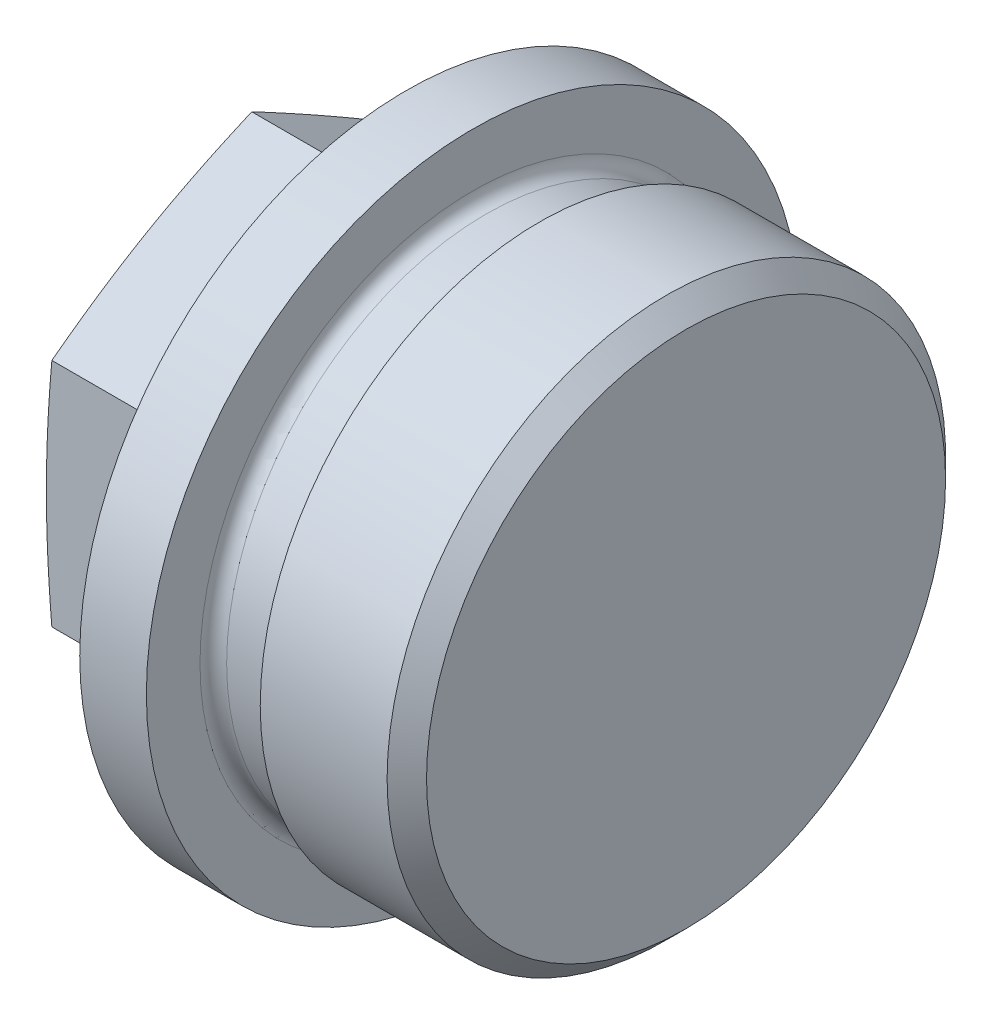
from build123d import *

# Parameters (mm, degrees)
EXTRUDE1_DEPTH     = 12
SKETCH3_OUTSIDE_W  = 179.776
SKETCH3_OUTSIDE_H  = 179.776
SKETCH3_OUTSIDE_R  = 15
CUT_EXTRUDE1_DEPTH = 10
CUT_EXTRUDE1_DRAFT = -80
FILLET1_R          = 1


with BuildPart() as part:
    # Sketch1 → Revolve1 (revolve)
    with BuildSketch(Plane.XY, mode=Mode.PRIVATE) as revolve1_sk:
        Polygon((22, 20.955), (22, 19.476), (17, 19.476), (17, 24.5), (12, 24.5), (12, 1.5), (0, 1.5), (0, 0), (33, 0), (33, 19.476), (31.521, 20.955), align=None)
    revolve(revolve1_sk.sketch.rotate(Axis((0, 0, 0), (1, 0, 0)), 90), axis=Axis((0, 0, 0), (1, 0, 0)))

    # Sketch2 → Extrude1 (add)
    with BuildSketch(Plane.ZY):
        Polygon((0, 17.320508076), (-15, 8.660254038), (-15, -8.660254038), (0, -17.320508076), (15, -8.660254038), (15, 8.660254038), align=None)
    extrude(amount=-EXTRUDE1_DEPTH)


with BuildPart() as cut_extrude1_tool:
    # Sketch3 outside → Cut-Extrude1 (with draft: the straight prism first)
    with BuildSketch(Plane.ZY):
        Rectangle(SKETCH3_OUTSIDE_W, SKETCH3_OUTSIDE_H)
        Circle(SKETCH3_OUTSIDE_R, mode=Mode.SUBTRACT)
    extrude(amount=-CUT_EXTRUDE1_DEPTH)
    # Cut-Extrude1: the draft: its side faces are tilted about the plane it starts from
    cut_extrude1_sides = [cut_extrude1_tool.faces().sort_by_distance(p)[0] for p in [
        (5, -89.888, 0),
        (5, 0, 89.888),
        (5, 89.888, 0),
        (5, 0, -89.888),
        (5, 0, -15),
    ]]
    draft(cut_extrude1_sides, Plane.ZY, CUT_EXTRUDE1_DRAFT)


with BuildPart() as part_1:
    add(part.part)

    # Cut-Extrude1: cut by cut_extrude1_tool
    add(cut_extrude1_tool.part, mode=Mode.SUBTRACT)

    # Fillet1
    fillet1_edges = [part_1.edges().sort_by_distance(p)[0] for p in [
        (22, 0, -19.476),
        (17, 0, -19.476),
    ]]
    fillet(fillet1_edges, radius=FILLET1_R)


solid = part_1.part
